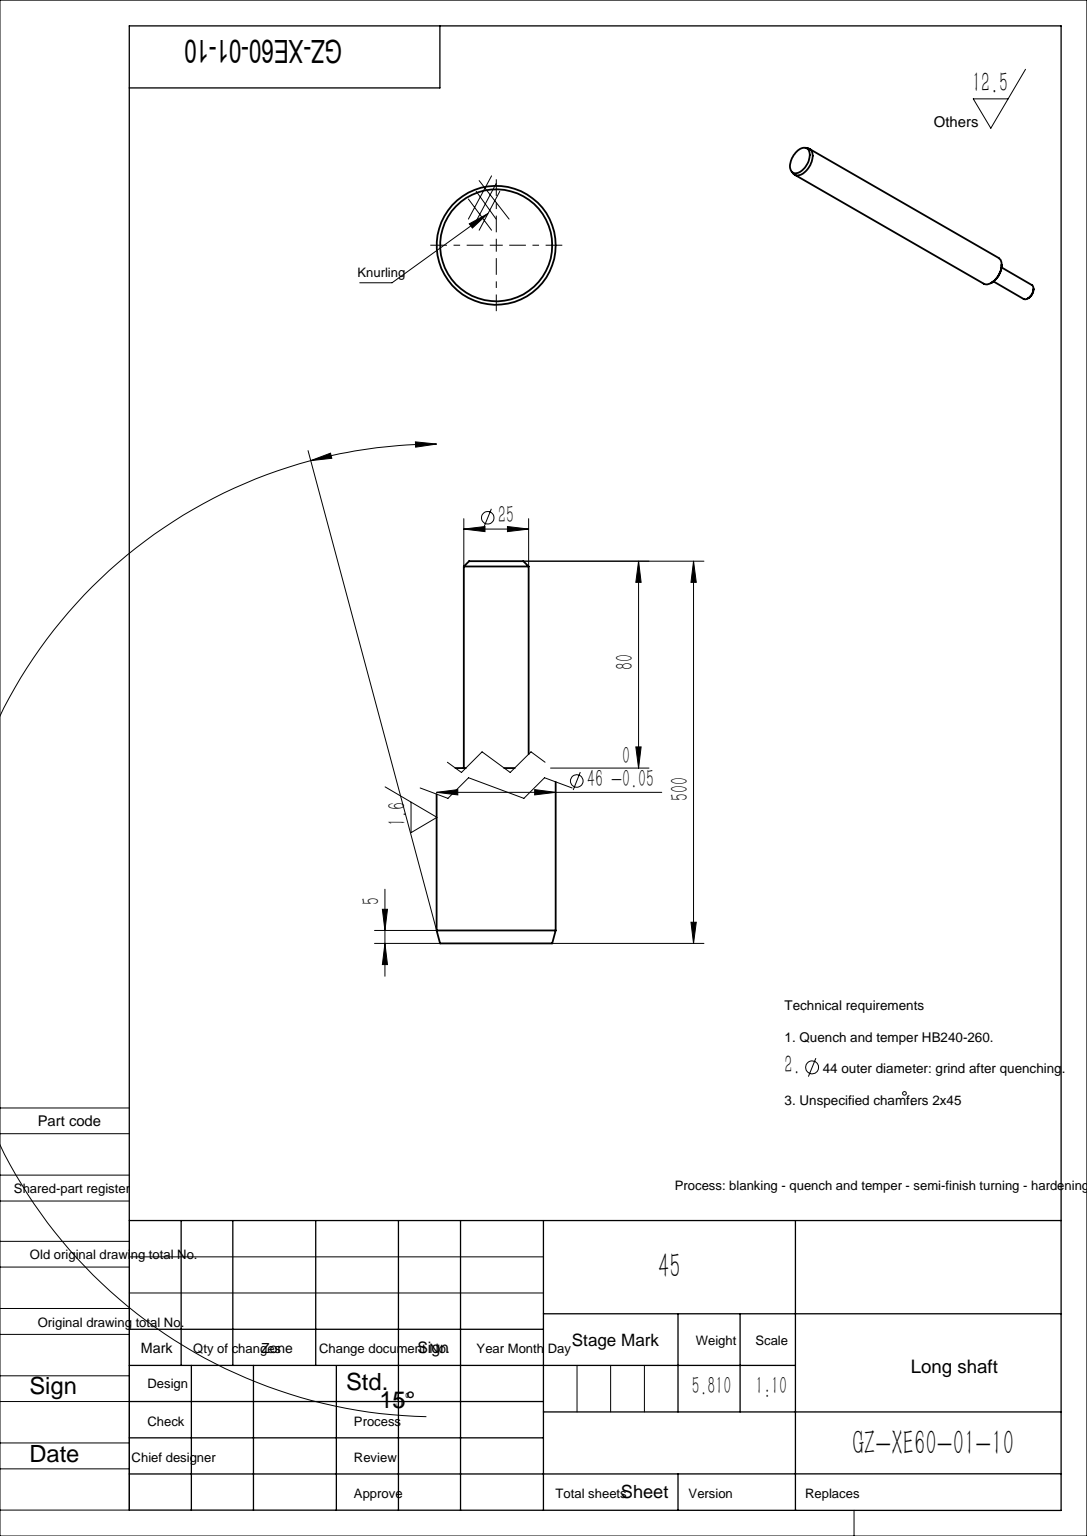
from build123d import *

# Parameters (mm, degrees)
SKETCH1_R           = 23
BOSS_EXTRUDE1_DEPTH = 420
CHAMFER1_SIZE       = 5
CHAMFER1_SIZE2      = 1.339745962
SKETCH2_R           = 12.5
BOSS_EXTRUDE2_DEPTH = 80
CHAMFER2_SIZE       = 2


with BuildPart() as part:
    # Sketch1 → Boss-Extrude1 (new body)
    with BuildSketch(Plane.XY):
        Circle(SKETCH1_R)
    extrude(amount=BOSS_EXTRUDE1_DEPTH)

    # Chamfer1
    chamfer1_edges = [part.edges().sort_by_distance(p)[0] for p in [
        (-23, 0, 420),
    ]]
    chamfer1_side = [part.faces().sort_by_distance(p)[0] for p in [
        (-23, 0, 210),
    ]]
    chamfer(chamfer1_edges, length=CHAMFER1_SIZE, length2=CHAMFER1_SIZE2, reference=chamfer1_side[0])

    # Sketch2 → Boss-Extrude2 (add)
    with BuildSketch(Plane(origin=(0, 0, 0), x_dir=(-1, 0, 0), z_dir=(0, 0, -1))):
        with Locations(Location((0, 0, 0), (0, 0, 180))):
            Circle(SKETCH2_R)
    extrude(amount=BOSS_EXTRUDE2_DEPTH)

    # Chamfer2
    chamfer2_edges = [part.edges().sort_by_distance(p)[0] for p in [
        (-23, 0, 0),
        (-12.5, 0, -80),
    ]]
    chamfer(chamfer2_edges, length=CHAMFER2_SIZE)


solid = part.part
